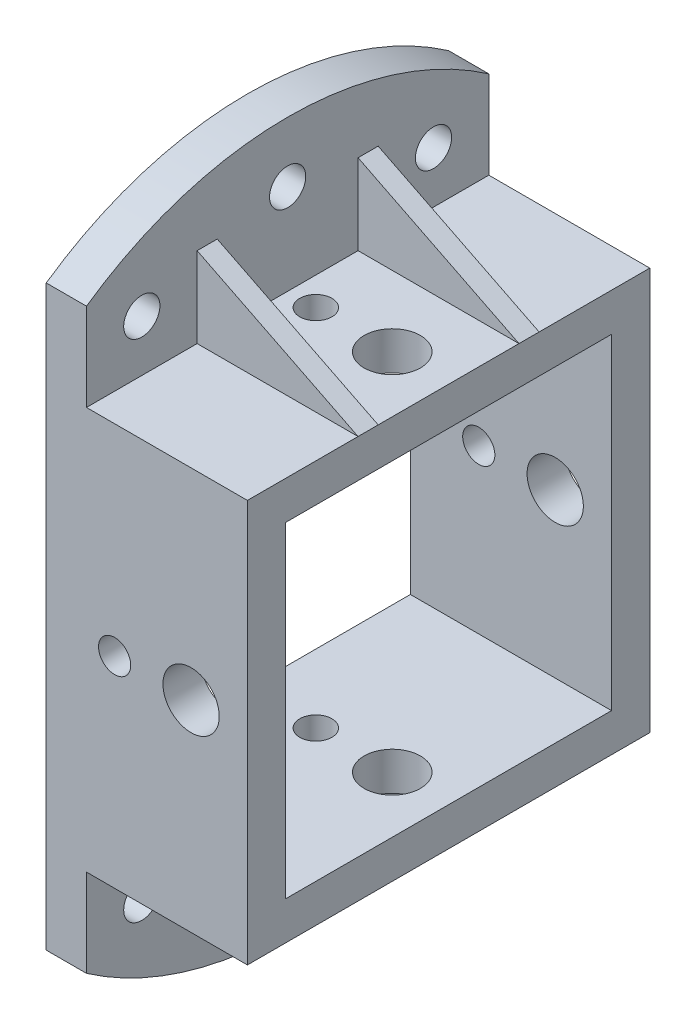
from build123d import *

# Parameters (mm, degrees)
SKETCH4_W               = 100
SKETCH4_H               = 100
SKETCH4_W_2             = 81
SKETCH4_H_2             = 81
BOSS_EXTRUDE1_DEPTH     = 40
SKETCH5_R               = 87.5
BOSS_EXTRUDE2_DEPTH     = 10
SKETCH6_OUTSIDE_W       = 227.498
SKETCH6_OUTSIDE_H       = 227.498
SKETCH6_OUTSIDE_W_2     = 100
SKETCH6_OUTSIDE_H_2     = 212.75110477
CUT_EXTRUDE1_DEPTH      = 10
SKETCH7_W               = 81
SKETCH7_H               = 81
CUT_EXTRUDE2_DEPTH      = 10
SKETCH8_R               = 4.5
CUT_EXTRUDE3_DEPTH      = 10
M16_TAPPED_HOLE1_D      = 14
M16_TAPPED_HOLE2_D      = 14
SIZE_MM_DOWEL_HOLE2_D   = 8
MM_2_D                  = 8
RIB2_REACH              = 120.98
SKETCH18_WALL_W         = 284.681440236
SKETCH18_WALL_H         = 5
MIRROR2_COPY_1_REACH    = 120.98
MIRROR2_COPY_1_SKETCH_W = 284.681440236
MIRROR2_COPY_1_SKETCH_H = 5


with BuildPart() as part:
    # Sketch4 → Boss-Extrude1 (new body)
    with BuildSketch(Plane(origin=(0, 0, 0), x_dir=(0, 0, -1), z_dir=(1, 0, 0))):
        Rectangle(SKETCH4_W, SKETCH4_H)
        Rectangle(SKETCH4_W_2, SKETCH4_H_2, mode=Mode.SUBTRACT)
    extrude(amount=BOSS_EXTRUDE1_DEPTH)

    # Sketch5 → Boss-Extrude2 (add)
    with BuildSketch(Plane.ZY):
        Circle(SKETCH5_R)
    extrude(amount=BOSS_EXTRUDE2_DEPTH)

    # Sketch6 outside → Cut-Extrude1 (cut)
    with BuildSketch(Plane.ZY.offset(10)):
        Rectangle(SKETCH6_OUTSIDE_W, SKETCH6_OUTSIDE_H)
        Rectangle(SKETCH6_OUTSIDE_W_2, SKETCH6_OUTSIDE_H_2, mode=Mode.SUBTRACT)
    extrude(amount=-CUT_EXTRUDE1_DEPTH, mode=Mode.SUBTRACT)

    # Sketch7 → Cut-Extrude2 (cut)
    with BuildSketch(Plane(origin=(0, 0, 0), x_dir=(0, 0, -1), z_dir=(1, 0, 0))):
        Rectangle(SKETCH7_W, SKETCH7_H)
    extrude(amount=-CUT_EXTRUDE2_DEPTH, mode=Mode.SUBTRACT)

    # Sketch8 → Cut-Extrude3 (cut)
    with BuildSketch(Plane(origin=(0, 0, 0), x_dir=(0, 0, -1), z_dir=(1, 0, 0))):
        with Locations((-36.25, 62.786841774)):
            Circle(SKETCH8_R)
        with Locations((0, 72.5)):
            Circle(SKETCH8_R)
        with Locations((36.25, 62.786841774)):
            Circle(SKETCH8_R)
        with Locations(Location((36.25, -62.786841774, 0), (0, 0, 180))):
            Circle(SKETCH8_R)
        with Locations(Location((0, -72.5, 0), (0, 0, 180))):
            Circle(SKETCH8_R)
        with Locations(Location((-36.25, -62.786841774, 0), (0, 0, 180))):
            Circle(SKETCH8_R)
    extrude(amount=-CUT_EXTRUDE3_DEPTH, mode=Mode.SUBTRACT)

    # M16 Tapped Hole1 (through all)
    with Locations(Plane.XY.offset(50)):
        with Locations((26, 0)):
            Hole(M16_TAPPED_HOLE1_D / 2)

    # M16 Tapped Hole2 (through all)
    with Locations(Plane(origin=(0, 50, 0), x_dir=(1, 0, 0), z_dir=(0, 1, 0))):
        with Locations((26, 0)):
            Hole(M16_TAPPED_HOLE2_D / 2)

    # Size mm Dowel Hole2 (through all)
    with Locations(Plane.XY.offset(50)):
        with Locations((7, 0)):
            Hole(SIZE_MM_DOWEL_HOLE2_D / 2)

    # 大小mm 暗销孔2 (through all)
    with Locations(Plane(origin=(0, 50, 0), x_dir=(1, 0, 0), z_dir=(0, 1, 0))):
        with Locations((7, 0)):
            Hole(MM_2_D / 2)

    # Sketch18 wall → Rib2 (add, up to next)
    with BuildSketch(Plane(origin=(20, 60, 20), x_dir=(-0.894427191, 0.4472135955, 0), z_dir=(-0.4472135955, -0.894427191, 0)), mode=Mode.PRIVATE) as rib2_sk1:
        Rectangle(SKETCH18_WALL_W, SKETCH18_WALL_H)
    rib2_tool1 = extrude(rib2_sk1.sketch, amount=RIB2_REACH, mode=Mode.PRIVATE) - part.part
    rib2 = rib2_tool1.solids().sort_by_distance((20, 60, 20))[0]
    add(rib2)

    # Mirror1: Rib2 across plane
    add(rib2.mirror(Plane.ZX))

    # Mirror2: Rib2 across plane
    add(rib2.mirror(Plane.XY))

    # Mirror2 copy 1 sketch → Mirror2 copy 1 (add, up to next)
    with BuildSketch(Plane(origin=(20, -60, -20), x_dir=(-0.894427191, -0.4472135955, 0), z_dir=(-0.4472135955, 0.894427191, 0)), mode=Mode.PRIVATE) as mirror2_copy_1_sk1:
        Rectangle(MIRROR2_COPY_1_SKETCH_W, MIRROR2_COPY_1_SKETCH_H)
    mirror2_copy_1_tool1 = extrude(mirror2_copy_1_sk1.sketch, amount=MIRROR2_COPY_1_REACH, mode=Mode.PRIVATE) - part.part
    add(mirror2_copy_1_tool1.solids().sort_by_distance((20, -60, -20))[0])


solid = part.part
